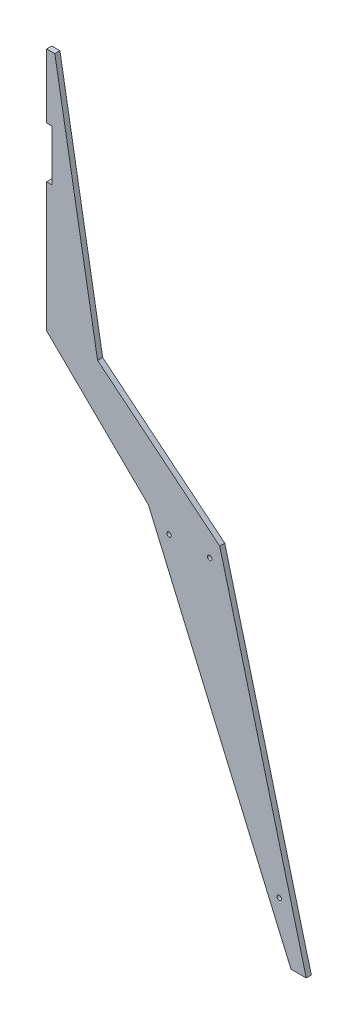
from build123d import *

# Parameters (mm, degrees)
EXTRUDE_1_DEPTH     = 2.5
SKETCH_2_R          = 2.2
CUT_EXTRUDE_1_DEPTH = 10
SKETCH_3_R          = 2.2
CUT_EXTRUDE_2_DEPTH = 10


with BuildPart() as part:
    # 草图1 → 凸台-拉伸1 (new, symmetric)
    with BuildSketch(Plane.XY):
        Polygon((0, 0), (8, 0), (50, -240), (170, -338), (255, -663), (240, -663), (100, -338), (0, -240), (0, -113), (5, -113), (5, -63), (0, -63), align=None)
    extrude(amount=EXTRUDE_1_DEPTH, both=True)

    # 草图2 → 切除-拉伸1 (cut)
    with BuildSketch(Plane.XY.offset(2.5)):
        with Locations((120.192307692, -353)):
            Circle(SKETCH_2_R)
        with Locations((160.192307692, -353)):
            Circle(SKETCH_2_R)
    extrude(amount=-CUT_EXTRUDE_1_DEPTH, mode=Mode.SUBTRACT)

    # 草图3 → 切除-拉伸2 (cut)
    with BuildSketch(Plane.XY.offset(2.5)):
        with Locations((228.461538462, -608)):
            Circle(SKETCH_3_R)
    extrude(amount=-CUT_EXTRUDE_2_DEPTH, mode=Mode.SUBTRACT)


solid = part.part
